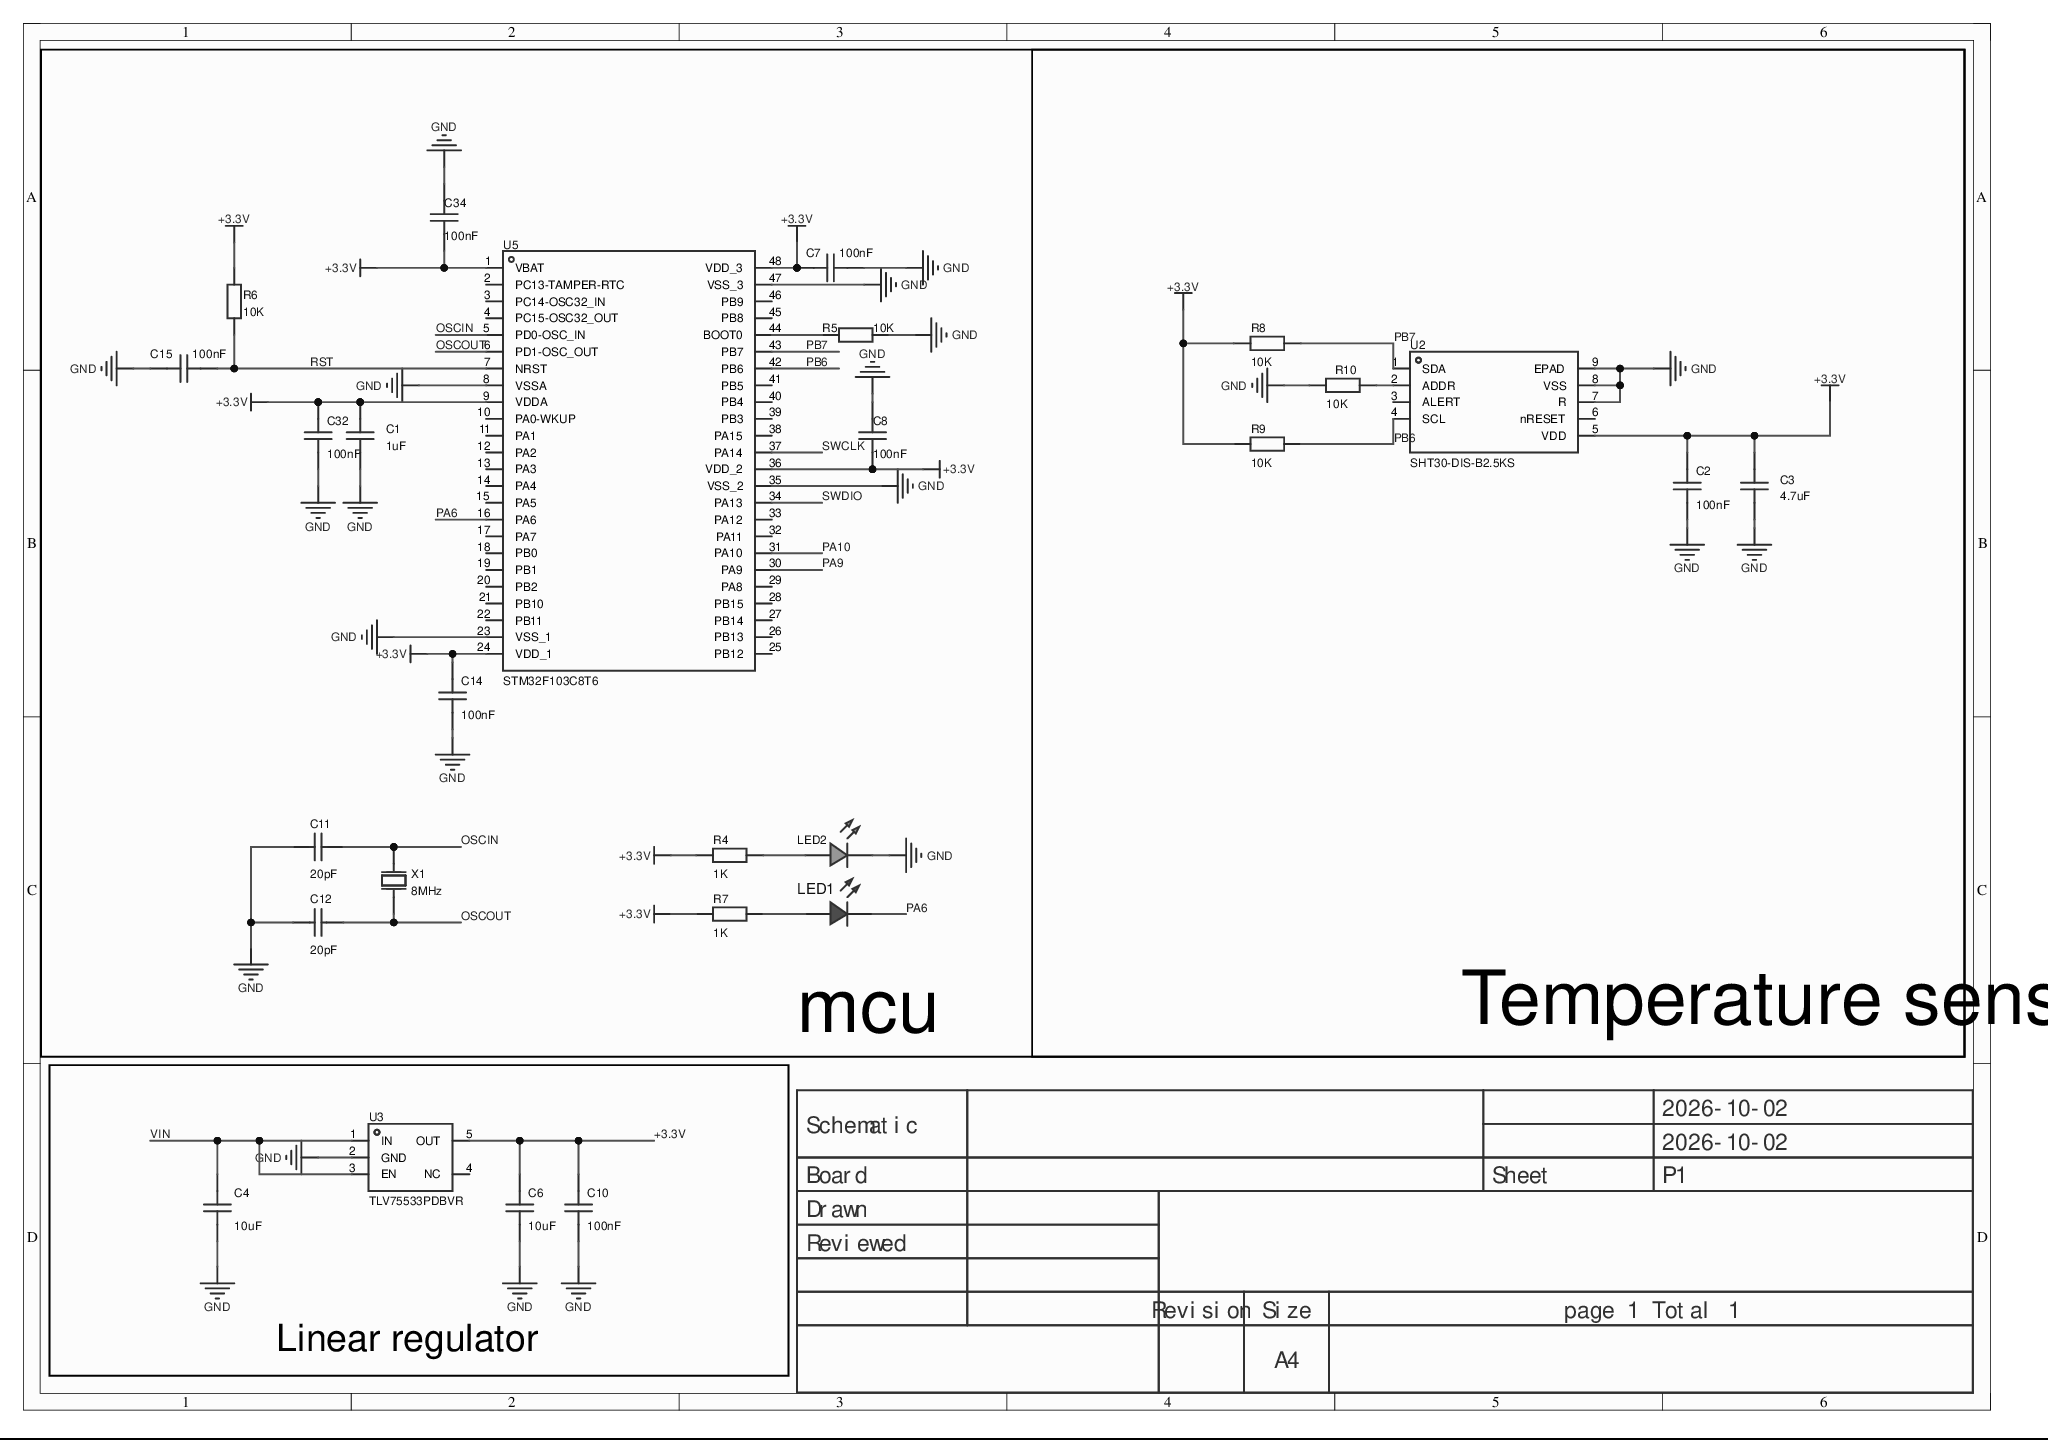
[diagram p0: MISC80717-2.schdoc]
# Altium schematic sheet MISC80717-2.schdoc
size 297 x 209 mm; Version: V1.0; @Project Name: MISC80717; @Update Date: 2026-10-02; @Create Date: 2026-10-02; @Board Name: MISC80717; @Create Time: 10:50:36; @Page Count: 1; @Page No: 1; @Schematic Name: MISC80717; @Update Time: 10:50:36; Size: A4

## Parts
C1  1uF  [C0603]
C2  100nF  [C0603]
C3  4.7uF  [C0805]
C4  10uF  [C0603]
C6  10uF  [C0603]
C7  100nF  [C0603]
C8  100nF  [C0603]
C10  100nF  [C0603]
C11  20pF  [C0603]
C12  20pF  [C0603]
C14  100nF  [C0603]
C15  100nF  [C0603]
C32  100nF  [C0603]
C34  100nF  [C0603]
LED1  (no value)  [LED_0603]
LED2  (no value)  [LED_0603]
R4  1K  [R0603]
R5  10K  [R0603]
R6  10K  [R0603]
R7  1K  [R0603]
R8  10K  [R0603]
R9  10K  [R0603]
R10  10K  [R0603]
U2  SHT30-DIS-B2.5KS  [DFN-8_L2.5-W2.5-P0.50-BL-EP]
U3  TLV75533PDBVR  [SOT-23-5_L3.0-W1.7-P0.95-LS2.8-BR]
U5  STM32F103C8T6  [LQFP-48_L7.0-W7.0-P0.50-LS9.0-BL]
X1  8MHz  [CRYSTAL-SMD_L5.0-W3.2]

## Blocks framed on the sheet
mcu: C1 C7 C8 C11 C12 C14 C15 C32 C34 LED1 LED2 R4-R7 U5 X1
Temperature sensor: C2 C3 R8-R10 U2
Linear regulator: C4 C6 C10 U3

## Nets
+3.3V: C1.2 C2.1 C3.2 C6.1 C7.2 C8.1 C10.2 C14.1 C32.2 C34.1 R4.1 R6.2 R7.1 R8.2 R9.2 U2.5(VDD) U3.5(OUT) U5.1(VBAT) U5.9(VDDA) U5.24(VDD_1) U5.36(VDD_2) U5.48(VDD_3)
GND: C1.1 C2.2 C3.1 C4.1 C6.2 C7.1 C8.2 C10.1 C11.1 C12.1 C14.2 C15.2 C32.1 C34.2 LED2.1(C) R5.2 R10.2 U2.7(R) U2.8(VSS) U2.9(EPAD) U3.2(GND) U5.8(VSSA) U5.23(VSS_1) U5.35(VSS_2) U5.47(VSS_3)
OSCIN: C11.2 U5.5(PD0-OSC_IN) X1.2(OSC2)
OSCOUT: C12.2 U5.6(PD1-OSC_OUT) X1.1(OSC1)
PA6: LED1.1(C) U5.16(PA6)
PA9: U5.30(PA9)
PA10: U5.31(PA10)
PB6: R9.1 U2.4(SCL) U5.42(PB6)
PB7: R8.1 U2.1(SDA) U5.43(PB7)
RST: C15.1 R6.1 U5.7(NRST)
SWCLK: U5.37(PA14)
SWDIO: U5.34(PA13)
VIN: C4.2 U3.1(IN) U3.3(EN)
NetLED1_2: LED1.2(A) R7.2
NetLED2_2: LED2.2(A) R4.2
NetR5_1: R5.1 U5.44(BOOT0)
NetR10_1: R10.1 U2.2(ADDR)

Not connected (* = marked no-connect by the designer): U2 3(ALERT)* 6(nRESET)*; U3 4(NC)*; U5 2(PC13-TAMPER-RTC)* 3(PC14-OSC32_IN)* 4(PC15-OSC32_OUT)* 10(PA0-WKUP)* 11(PA1)* 12(PA2)* 13(PA3)* 14(PA4)* 15(PA5)* 17(PA7)* 18(PB0)* 19(PB1)* 20(PB2)* 21(PB10)* 22(PB11)* 25(PB12)* 26(PB13)* 27(PB14)* 28(PB15)* 29(PA8)* 32(PA11)* 33(PA12)* 38(PA15)* 39(PB3)* 40(PB4)* 41(PB5)* 45(PB8)* 46(PB9)*

## Notes on the sheet
- 2026-10-02
- Schematic
- Board
- Sheet
- P1
- Drawn
- Reviewed
- Revision
- Size
- A4
- page 1 Total 1

## Library data of the parts
C1 = CL10A105KB8NNNC: Capacitance:1uF;Accuracy:±10%;Rated voltage:50V;Temperature coefficient:X5R;; Manufacturer: SAMSUNG(三星); AddInBom: yes; ModelId: ac125912035d415993ca9572d50418b10819f05c4eef4c71ace90d822a990e87; ModelName: C0603_L1.6-W0.8-H0.8; ModelTransform: 62.992,31.496,0,0,0,0,0,0,0; Tolerance: ±10%; Voltage Rating: 50V; Temperature Coefficient: X5R; Symbol: CL10A105KB8NNNC; Device: CL10A105KB8NNNC; LCSC Part Name: 1uF ±10% 50V; SupplierPart: C15849; ManufacturerPart: CL10A105KB8NNNC; Supplier Footprint: 0603; JLCPCB Part Class: Basic Part; Datasheet: example.com/datasheet/CL10A105KB8NNNC/16531.html; Supplier: LCSC; ConvertToPcb: yes; FootprintName: C0603; Value: 1uF
C2 C7 C8 C10 C14 C15 = CGA0603X7R104K500JT: Capacitance:100nF;Accuracy:±10%;Rated voltage:50V;Temperature coefficient:X7R;; Manufacturer: HRE(芯声); 3D Model: ac125912035d415993ca9572d50418b10819f05c4eef4c71ace90d822a990e87; 3D Model Transform: 62.992,31.496,0,0,0,0,0,0,0; Tolerance: ±10%; Voltage Rating: 50V; Temperature Coefficient: X7R; AddInBom: yes; ModelName: C0603_L1.6-W0.8-H0.8; Symbol: CGA0603X7R104K500JT; Device: CGA0603X7R104K500JT; LCSC Part Name: 100nF ±10% 50V; Supplier Part: C6119867; Manufacturer Part: CGA0603X7R104K500JT; Supplier Footprint: 0603; JLCPCB Part Class: Extended Part; Datasheet: example.com/datasheet/CGA0603X7R104K500JT/7062573.html; Supplier: LCSC; Value: 100nF; ConvertToPcb: yes; FootprintName: C0603
C3 = HGC0805R7475K500NSLJ: Capacitance:4.7uF;Accuracy:±10%;Rated voltage:50V;Temperature coefficient:X7R;; Manufacturer: Chinocera(华瓷); AddInBom: yes; ModelId: 1ba041120af144c991958decab20d2410819f05c4eef4c71ace90d822a990e87; ModelName: C0805_L2.0-W1.3-H1.3; ModelTransform: 78.74,51.181,0,0,0,0,0,0.0005,0; Tolerance: ±10%; Voltage Rating: 50V; Temperature Coefficient: X7R; Symbol: HGC0805R7475K500NSLJ; Device: HGC0805R7475K500NSLJ; LCSC Part Name: 4.7uF ±10% 50V; SupplierPart: C7472970; ManufacturerPart: HGC0805R7475K500NSLJ; Supplier Footprint: 0805; JLCPCB Part Class: Extended Part; Datasheet: example.com/datasheet/HGC0805R7475K500NSLJ/8532817.html; Supplier: LCSC; ConvertToPcb: yes; FootprintName: C0805; Value: 4.7uF
C4 C6 = HGC0603R5106M160NTHJ: Capacitance:10uF;Accuracy:±20%;Rated voltage:16V;Temperature coefficient:X5R;; Manufacturer: Chinocera(华瓷); AddInBom: yes; ModelId: ac125912035d415993ca9572d50418b10819f05c4eef4c71ace90d822a990e87; ModelName: C0603_L1.6-W0.8-H0.8; ModelTransform: 62.992,31.496,0,0,0,0,0,0,0; Tolerance: ±20%; Voltage Rating: 16V; Temperature Coefficient: X5R; Symbol: HGC0603R5106M160NTHJ; Device: HGC0603R5106M160NTHJ; LCSC Part Name: 10uF ±20% 16V; SupplierPart: C7472959; ManufacturerPart: HGC0603R5106M160NTHJ; Supplier Footprint: 0603; JLCPCB Part Class: Extended Part; Datasheet: example.com/datasheet/HGC0603R5106M160NTHJ/8532806.html; Supplier: LCSC; ConvertToPcb: yes; FootprintName: C0603; Value: 10uF
C11 C12 = CL10C200JB8NNNC: Capacitance:20pF;Accuracy:±5%;Rated voltage:50V;Temperature coefficient:C0G;; Manufacturer: SAMSUNG(三星); AddInBom: yes; ModelId: ac125912035d415993ca9572d50418b10819f05c4eef4c71ace90d822a990e87; ModelName: C0603_L1.6-W0.8-H0.8; ModelTransform: 62.992,31.496,0,0,0,0,0,0,0; Tolerance: ±5%; Voltage Rating: 50V; Temperature Coefficient: C0G; Symbol: CL10C200JB8NNNC; Device: CL10C200JB8NNNC; LCSC Part Name: 20pF ±5% 50V; SupplierPart: C1648; ManufacturerPart: CL10C200JB8NNNC; Supplier Footprint: 0603; JLCPCB Part Class: Basic Part; Datasheet: example.com/datasheet/CL10C200JB8NNNC/2000.html; Supplier: LCSC; ConvertToPcb: yes; FootprintName: C0603; Value: 20pF
C32 C34 = CAP_0603: Symbol: Capacitance; 3D Model: ac125912035d415993ca9572d50418b10819f05c4eef4c71ace90d822a990e87; 3D Model Transform: 62.992,31.496,0,0,0,0,0,0,0; ConvertToPcb: yes; ModelName: C0603_L1.6-W0.8-H0.8; Device: CAP_0603; Supplier Footprint: 0603; Value: 100nF; AddInBom: yes; FootprintName: C0603
LED1 = LED_0603-R: Symbol: LED_R; Convert to PCB: yes; 3D Model: dd8257b0d61a4cd7b68939a056e080950819f05c4eef4c71ace90d822a990e87; 3D Model Transform: 58.72,29.4,22.03,0,0,0,0,0,0; ModelName: LED-0603_R; Device: LED_0603-R; Add into BOM: yes; Supplier Footprint: 0603; FootprintName: LED_0603
LED2 = LED_0603-G: Symbol: LED_G_OLD; Convert to PCB: yes; 3D Model: 8b5fcaf0229049f8a37a9c352bb0ca0a0819f05c4eef4c71ace90d822a990e87; 3D Model Transform: 63.1,31.6,23.7,0,0,0,0,0,0; ModelName: LED-0603_G; Device: LED_0603-G; Add into BOM: yes; Supplier Footprint: 0603; FootprintName: LED_0603
R4-R10 = Res_0603: Symbol: Resistor; 3D Model: fc143cca1e79419f9cd78b61e9279f080819f05c4eef4c71ace90d822a990e87; 3D Model Transform: 31.8897,63.7794,0,90,0,0,0,0,0; ConvertToPcb: yes; Device: Res_0603; Supplier Footprint: 0603; AddInBom: yes; FootprintName: R0603; ModelName: R0603
  R4 R7: Value: 1K
  R5 R6 R8-R10: Value: 10K
U2 = SHT30-DIS-B2.5KS: Temperature range:-40℃~+125℃;Humidity range:0%RH~100%RH;Interface type:I2C;Humidity accuracy:±2%RH;; Manufacturer: Sensirion(瑞士盛思锐); AddInBom: yes; ModelId: bc1ff5dd6aff4b369d2fdcf934ef0d2a0819f05c4eef4c71ace90d822a990e87; ModelName: DFN-8_L2.5-W2.5-H1.0-P0.50; ModelTransform: 99.2124,98.425,0,90,0,0,-0.003,-0.003,0; Interface: I2C; Voltage - Supply: 2.15V~5.5V; Current - Supply: 200nA; Humidity Tolerance: ±2%RH; Temperature Tolerance: ±0.2℃; Resolution: 16bit; Symbol: SHT30-DIS-B; Device: SHT30-DIS-B2.5KS; LCSC Part Name: 1-101400-01 1-101400-01 ±2%数字温湿度传感器（10-90%RH）; SupplierPart: C77361; ManufacturerPart: SHT30-DIS-B2.5KS; Supplier Footprint: DFN-8-EP(2.5x2.5); JLCPCB Part Class: Extended Part; Datasheet: example.com/datasheet/SHT30-DIS-B2.5KS/78489.html; Supplier: LCSC; ConvertToPcb: yes; FootprintName: DFN-8_L2.5-W2.5-P0.50-BL-EP; Temperature Range: -40℃~+125℃; Humidity: 0%RH~100%RH; Features: Temperature compensation; factory calibration
U3 = TLV75533PDBVR: Output polarity:Positive;Operating voltage:5.5V;Output voltage:3.3V;Output current:500mA;Power supply rejection ratio (PSRR):46dB@(100kHz);Output type:Fixed;; Manufacturer: TI(德州仪器); AddInBom: yes; ModelId: 0a2a1b8f50944f73965918ad6e5fe1670819f05c4eef4c71ace90d822a990e87; ModelName: SOT-23-5_L2.9-W1.6-H1.1-LS2.8-P0.95; ModelTransform: 114.173,109.636,0,180,0,0,0,0,0; Voltage - Supply: 5.5V; Output Voltage: 3.3V; Output Current: 500mA; Voltage Dropout: 238mV@(500mA); standby current: 25uA; Noise: 71.5uVrms; Output Type: Fixed; Number of Outputs: 1; Symbol: TLV75533PDBVR; Device: TLV75533PDBVR; LCSC Part Name: 3.3V 500mA 5.5V; SupplierPart: C404027; ManufacturerPart: TLV75533PDBVR; Supplier Footprint: SOT-23-5; JLCPCB Part Class: Extended Part; Datasheet: example.com/cn/lit/ds/symlink/tlv755p.pdf; Supplier: LCSC; ConvertToPcb: yes; FootprintName: SOT-23-5_L3.0-W1.7-P0.95-LS2.8-BR; Output Configuration: Positive; Power Supply Rejection Ratio (PSRR): 46dB@(100kHz); Features: Enable control; output discharge; built-in soft start; short-circuit protection; overcurrent protection; thermal shutdown; input undervoltage protection; Operating Temperature: -40℃~+125℃@(Tj)
U5 = STM32F103C8T6: CPU core:ARM-M3;Max CPU frequency:72MHz;Application field:-;; Manufacturer: ST(意法半导体); 3D Model: 093be70396ff421eb2cdb946d5311efc0819f05c4eef4c71ace90d822a990e87; 3D Model Transform: 354.331,354.331,0,0,0,0,0,0,0; CPU Core: ARM-M3; CPU Maximum Speed: 72MHz; Program Storage Size: 64KB; Program Memory Type: FLASH; Number of I/O: 37; ADC (Bit): 12bit; Voltage - Supply: 2V~3.6V; Core Size: 32 Bit; RAM Size: 20KB; Oscillator Type: Built-in; AddInBom: yes; ModelName: LQFP-48_L7.0-W7.0-H1.4-LS9.0-P0.50; Symbol: STM32F103C8T6; Device: STM32F103C8T6; LCSC Part Name: 主流增强型ARM Cortex-M3 MCU，具有64 KB Flash、72 MHz CPU、电机控制、USB和CAN; Supplier Part: C8734; Manufacturer Part: STM32F103C8T6; Supplier Footprint: LQFP-48(7x7); JLCPCB Part Class: Extended Part; Datasheet: example.com/datasheet/STM32F103C8T6/9243.html; Supplier: LCSC; Applications: -; EEPROM: -; Operating Temperature: -40℃~+85℃; ConvertToPcb: yes; FootprintName: LQFP-48_L7.0-W7.0-P0.50-LS9.0-BL
X1 = X50328MSB2GI: Crystal type:SMD crystal;Frequency:8MHz;Frequency tolerance at room temperature:±10ppm;Load capacitance:20pF;Frequency stability:±20ppm;; Manufacturer: YXC(扬兴晶振); 3D Model: d7c39c66443246ff83c2003c1e1eb6f10819f05c4eef4c71ace90d822a990e87; 3D Model Transform: 196.85,125.984,0,0,0,0,0,0,0; Normal temperature Frequency Tolerance: ±10ppm; Load Capacitance: 20pF; Frequency Stability: ±20ppm; Equivalent Series Resistance(ESR): 80Ω; AddInBom: yes; Symbol: X50328MSB2GI; Device: X50328MSB2GI; LCSC Part Name: YSX530GA 8MHZ 2P 5032 20PF ±10PPM -40~85℃ (±20PPM); Supplier Part: C115962; Manufacturer Part: X50328MSB2GI; Supplier Footprint: SMD5032-2P; JLCPCB Part Class: Basic Part; Datasheet: example.com/datasheet/X50328MSB2GI/117214.html; Supplier: LCSC; Type: SMD crystal; Value: 8MHz; Operating Temperature: -40℃~+85℃; ConvertToPcb: yes; FootprintName: CRYSTAL-SMD_L5.0-W3.2; ModelName: CRYSTAL-SMD_L5.0-W3.2